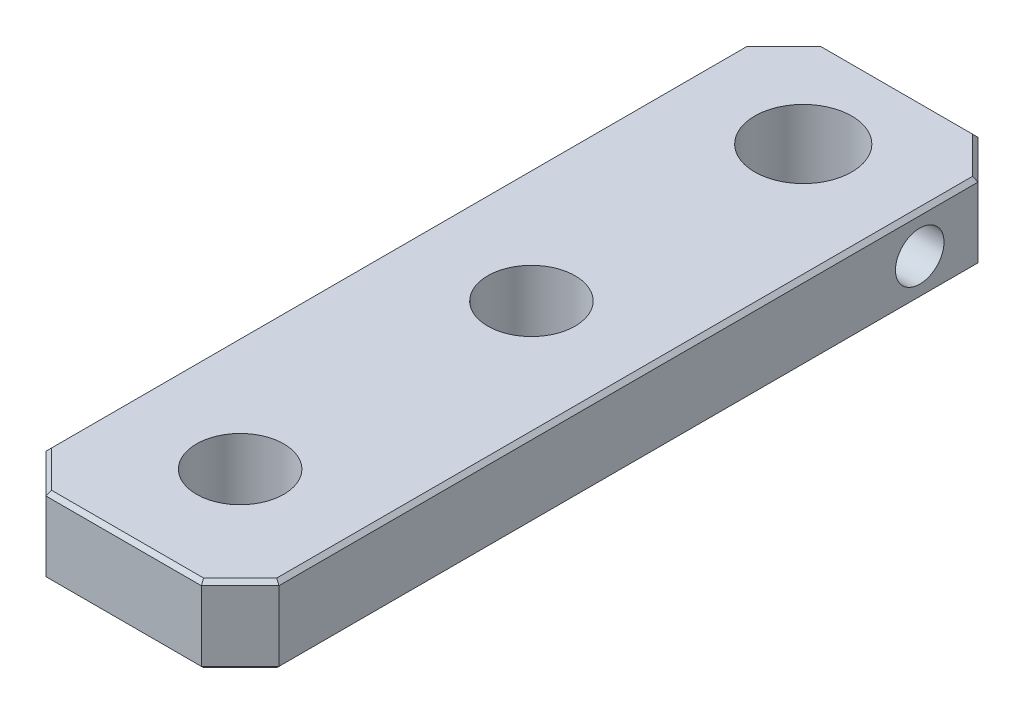
SolidWorks part; units mm, degrees
ref_plane "Front Plane" through (0, 0, 0) normal (0, 0, 1) x (1, 0, 0)
ref_plane "Top Plane" through (0, 0, 0) normal (0, 1, 0) x (1, 0, 0)
ref_plane "Right Plane" through (0, 0, 0) normal (1, 0, 0) x (0, 0, -1)
sketch "Sketch1" plane through (0, 0, 0) normal (0, 1, 0) x (1, 0, 0)
  line L1 (-6, 20) -> (6, 20)
  line L2 (-6, 20) -> (-6, -20)
  line L3 (-6, -20) -> (6, -20)
  line L4 (6, 20) -> (6, -20)
  line L5 (-6, 20) -> (6, -20) construction
  line L6 (-6, -20) -> (6, 20) construction
  point P0 (0, 0)
  dimension "D1" = 12
  dimension "D2" = 40
extrude "Boss-Extrude1" add sketch "Sketch1" along normal mid plane 4
chamfer "Chamfer1" distance 2 angle 45 4 edges at (-6, 0, -20) (6, 0, -20) (6, 0, 20) (-6, 0, 20)
hole_wizard "M6 Tapped Hole1" positions "Sketch3" profile "Sketch2" tap size "M6" standard "Gb" end condition through all
sketch "Sketch3" plane through (0, 2, 0) normal (0, 1, 0) x (1, 0, 0)
  line L1 (4, 20) -> (-4, 20) construction
  point P0 (0, 15)
  dimension "D1" = 5
sketch "Sketch2" plane through (0, 2, -15) normal (1, 0, 0) x (0, 0, 1)
  line L0 (0, 0) -> (0, 4)
  line L1 (0, 4) -> (2.5, 4)
  line L2 (2.5, 4) -> (2.5, 0)
  line L5 (2.5, 0) -> (0, 0)
  line L11 (0, -6.35) -> (0, 107.95) construction
  dimension "通孔螺纹孔钻头直径" = 5
  dimension "通孔螺纹孔钻头深度" = 4
cosmetic thread "Hole Thread1" parameters "D2"=6
hole_wizard "Ø4.5 (4.5) Diameter Hole1" positions "Sketch5" profile "Sketch4" hole size "Ø4.5" standard "Gb" end condition through all
sketch "Sketch5" plane through (0, 2, 0) normal (0, 1, 0) x (1, 0, 0)
  line L0 (-4, -20) -> (4, -20) construction
  point P0 (0, 1)
  point P2 (0, -14)
  dimension "D1" = 15
  dimension "D2" = 6
sketch "Sketch4" plane through (0, 2, -1) normal (1, 0, 0) x (0, 0, 1)
  line L0 (0, 0) -> (0, 4)
  line L1 (0, 4) -> (2.25, 4)
  line L2 (2.25, 4) -> (2.25, 0)
  line L5 (2.25, 0) -> (0, 0)
  line L11 (0, -6.35) -> (0, 107.95) construction
  dimension "通孔孔直径" = 4.5
  dimension "通孔孔深度" = 4
hole_wizard "M3 Tapped Hole1" positions "Sketch7" profile "Sketch6" tap size "M3" standard "Gb"
sketch "Sketch7" plane through (6, 0, 0) normal (1, 0, 0) x (0, 0, -1)
  line L0 (20, 2) -> (20, -2) construction
  point P0 (15, 0)
  dimension "D1" = 5
sketch "Sketch6" plane through (6, 0, -15) normal (0, 1, 0) x (0, 0, -1)
  line L0 (0, 0) -> (0, 3.5)
  line L1 (0, 3.5) -> (1.25, 3.5)
  line L2 (1.25, 3.5) -> (1.25, 0)
  line L5 (1.25, 0) -> (0, 0)
  line L11 (0, -6.35) -> (0, 107.95) construction
  dimension "通孔螺纹孔钻头直径" = 2.5
  dimension "通孔螺纹孔钻头深度" = 3.5
cosmetic thread "Hole Thread2" parameters "D2"=3
chamfer "Chamfer2" distance 0.2 angle 45 16 edges at (-6, -2, 0) (-6, 2, 0) (6, 2, 0) (6, -2, 0) (-5, 2, 19) (-5, 2, -19) (0, 2, -20) (5, 2, -19) (0, 2, 20) (5, 2, 19) (-5, -2, 19) (-5, -2, -19) (0, -2, -20) (5, -2, -19) (0, -2, 20) (5, -2, 19)
